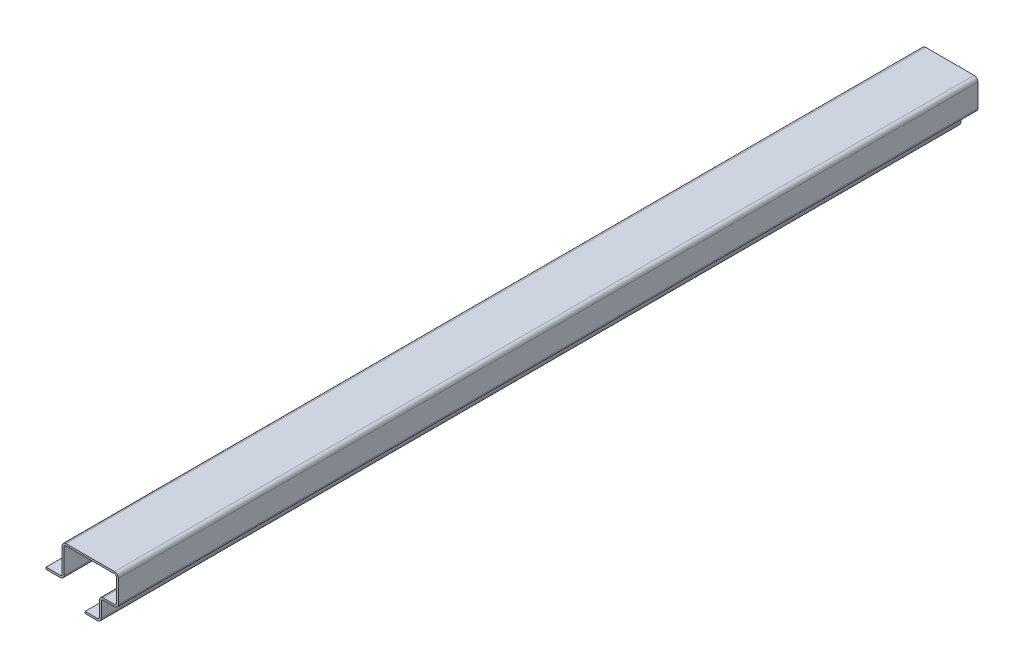
from build123d import *

# Parameters (mm, degrees)
BOSS_EXTRUDE1_DEPTH = 2660


with BuildPart() as part:
    # Sketch1 → Boss-Extrude1 (new body)
    with BuildSketch(Plane.XY):
        with BuildLine():
            Line((-70.999999998, 146), (-70.999999998, 70))
            ThreePointArc((-70.999999998, 70), (-72.757359311, 65.757359313), (-76.999999998, 64))
            Line((-76.999999998, 64), (-120.999999998, 64))
            Line((-120.999999998, 64), (-120.999999998, 58))
            Line((-120.999999998, 58), (-76.999999998, 58))
            ThreePointArc((-76.999999998, 58), (-68.514718624, 61.514718626), (-64.999999998, 70))
            Line((-64.999999998, 70), (-64.999999998, 146))
            ThreePointArc((-64.999999998, 146), (-63.242640685, 150.242640687), (-58.999999998, 152))
            Line((-58.999999998, 152), (91, 152))
            ThreePointArc((91, 152), (95.242640687, 150.242640687), (97, 146))
            Line((97, 146), (97, 76))
            ThreePointArc((97, 76), (95.242640687, 71.757359313), (91, 70))
            Line((91, 70), (56, 70))
            ThreePointArc((56, 70), (47.514718626, 66.485281374), (44, 58))
            Line((44, 58), (44, 12))
            ThreePointArc((44, 12), (42.242640687, 7.757359313), (38, 6))
            Line((38, 6), (0, 6))
            Line((0, 6), (0, 0))
            Line((0, 0), (38, 0))
            ThreePointArc((38, 0), (46.485281374, 3.514718626), (50, 12))
            Line((50, 12), (50, 58))
            ThreePointArc((50, 58), (51.757359313, 62.242640687), (56, 64))
            Line((56, 64), (91, 64))
            ThreePointArc((91, 64), (99.485281374, 67.514718626), (103, 76))
            Line((103, 76), (103, 146))
            ThreePointArc((103, 146), (99.485281374, 154.485281374), (91, 158))
            Line((91, 158), (-58.999999998, 158))
            ThreePointArc((-58.999999998, 158), (-67.485281372, 154.485281374), (-70.999999998, 146))
        make_face()
    extrude(amount=BOSS_EXTRUDE1_DEPTH)


solid = part.part
